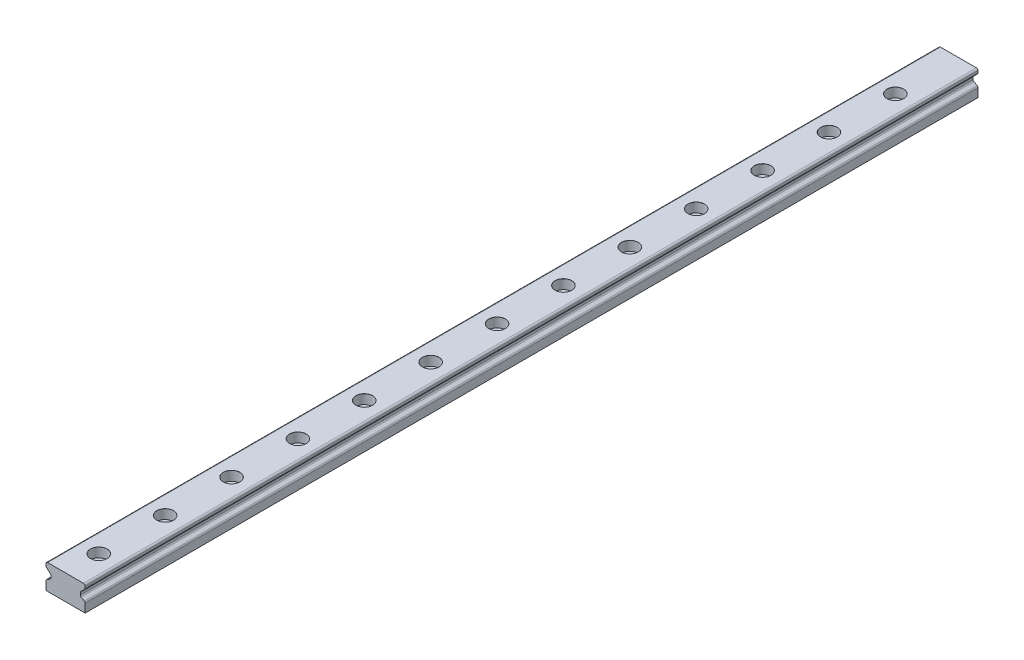
from build123d import *

# Parameters (mm, degrees)
BOSS_EXTRUDE1_DEPTH                           = 538
CBORE_FOR_M5_HEXAGON_SOCKET_HEAD_CAP_2_COUNT  = 2
CBORE_FOR_M5_HEXAGON_SOCKET_HEAD_CAP_2_PITCH  = 40
CBORE_FOR_M5_HEXAGON_SOCKET_HEAD_CAP_3_COUNT  = 2
CBORE_FOR_M5_HEXAGON_SOCKET_HEAD_CAP_3_PITCH  = 80
CBORE_FOR_M5_HEXAGON_SOCKET_HEAD_CAP_4_COUNT  = 2
CBORE_FOR_M5_HEXAGON_SOCKET_HEAD_CAP_4_PITCH  = 120
CBORE_FOR_M5_HEXAGON_SOCKET_HEAD_CAP_5_COUNT  = 2
CBORE_FOR_M5_HEXAGON_SOCKET_HEAD_CAP_5_PITCH  = 160
CBORE_FOR_M5_HEXAGON_SOCKET_HEAD_CAP_6_COUNT  = 2
CBORE_FOR_M5_HEXAGON_SOCKET_HEAD_CAP_6_PITCH  = 200
CBORE_FOR_M5_HEXAGON_SOCKET_HEAD_CAP_7_COUNT  = 2
CBORE_FOR_M5_HEXAGON_SOCKET_HEAD_CAP_7_PITCH  = 240
CBORE_FOR_M5_HEXAGON_SOCKET_HEAD_CAP_8_COUNT  = 2
CBORE_FOR_M5_HEXAGON_SOCKET_HEAD_CAP_8_PITCH  = 280
CBORE_FOR_M5_HEXAGON_SOCKET_HEAD_CAP_9_COUNT  = 2
CBORE_FOR_M5_HEXAGON_SOCKET_HEAD_CAP_9_PITCH  = 320
CBORE_FOR_M5_HEXAGON_SOCKET_HEAD_CAP_10_COUNT = 2
CBORE_FOR_M5_HEXAGON_SOCKET_HEAD_CAP_10_PITCH = 360
CBORE_FOR_M5_HEXAGON_SOCKET_HEAD_CAP_11_COUNT = 2
CBORE_FOR_M5_HEXAGON_SOCKET_HEAD_CAP_11_PITCH = 400
CBORE_FOR_M5_HEXAGON_SOCKET_HEAD_CAP_12_COUNT = 2
CBORE_FOR_M5_HEXAGON_SOCKET_HEAD_CAP_12_PITCH = 440
CBORE_FOR_M5_HEXAGON_SOCKET_HEAD_CAP_13_COUNT = 2
CBORE_FOR_M5_HEXAGON_SOCKET_HEAD_CAP_13_PITCH = 480


with BuildPart() as part:
    # Sketch1 → Boss-Extrude1 (new body)
    with BuildSketch(Plane.XY):
        with BuildLine():
            Line((-49.04910749, -219.573051322), (-49.04910749, -215.151654368))
            Line((-49.04910749, -215.151654368), (-49.04910749, -204.495232783))
            Line((-49.04910749, -204.495232783), (-59.847547756, -204.495232783))
            ThreePointArc((-59.847547756, -204.495232783), (-60.554654537, -204.788126002), (-60.847547756, -205.495232783))
            Line((-60.847547756, -205.495232783), (-60.847547756, -206.646526247))
            ThreePointArc((-60.847547756, -206.646526247), (-60.764684782, -207.045098292), (-60.529828406, -207.377616608))
            Line((-60.529828406, -207.377616608), (-58.226748647, -209.52693609))
            ThreePointArc((-58.226748647, -209.52693609), (-57.991892271, -209.859454405), (-57.909029297, -210.25802645))
            Line((-57.909029297, -210.25802645), (-57.909029297, -211.560962818))
            ThreePointArc((-57.909029297, -211.560962818), (-58.043527512, -212.061868659), (-58.410842619, -212.428032616))
            Line((-58.410842619, -212.428032616), (-60.345734434, -213.539750876))
            ThreePointArc((-60.345734434, -213.539750876), (-60.713049541, -213.905914833), (-60.847547756, -214.406820673))
            Line((-60.847547756, -214.406820673), (-60.847547756, -219.573051322))
            Line((-60.847547756, -219.573051322), (-49.04910749, -219.573051322))
        make_face()
        with BuildLine():
            Line((-49.04910749, -204.495232783), (-49.04910749, -215.151654368))
            Line((-49.04910749, -215.151654368), (-49.04910749, -219.573051322))
            Line((-49.04910749, -219.573051322), (-37.250667225, -219.573051322))
            Line((-37.250667225, -219.573051322), (-37.250667225, -214.406820673))
            ThreePointArc((-37.250667225, -214.406820673), (-37.38516544, -213.905914833), (-37.752480546, -213.539750876))
            Line((-37.752480546, -213.539750876), (-39.687372362, -212.428032616))
            ThreePointArc((-39.687372362, -212.428032616), (-40.054687468, -212.061868659), (-40.189185684, -211.560962818))
            Line((-40.189185684, -211.560962818), (-40.189185684, -210.25802645))
            ThreePointArc((-40.189185684, -210.25802645), (-40.10632271, -209.859454405), (-39.871466333, -209.52693609))
            Line((-39.871466333, -209.52693609), (-37.568386575, -207.377616608))
            ThreePointArc((-37.568386575, -207.377616608), (-37.333530198, -207.045098292), (-37.250667225, -206.646526247))
            Line((-37.250667225, -206.646526247), (-37.250667225, -205.495232783))
            ThreePointArc((-37.250667225, -205.495232783), (-37.543560443, -204.788126002), (-38.250667225, -204.495232783))
            Line((-38.250667225, -204.495232783), (-49.04910749, -204.495232783))
        make_face()
    extrude(amount=BOSS_EXTRUDE1_DEPTH)

    # Sketch3 → CBORE for M5 Hexagon socket head cap screws1 (revolve, cut)
    with BuildSketch(Plane(origin=(-49.04910749, -204.495232783, 518), x_dir=(0, 0, 1), z_dir=(1, 0, 0))):
        Polygon((0, 0), (0, 15.077818539), (2.75, 15.077818539), (2.75, 5.7), (5, 5.7), (5, 0.025), (5.025, 0), align=None)
    cbore_for_m5_hexagon_socket_head_cap_scr = revolve(axis=Axis((-49.04910749, -198.145232783, 518), (0, -1, 0)), mode=Mode.SUBTRACT)

    # CBORE for M5 Hexagon socket head cap 2: CBORE for M5 Hexagon socket head cap screws1 ×2
    with Locations(*[(0, 0, -i * CBORE_FOR_M5_HEXAGON_SOCKET_HEAD_CAP_2_PITCH) for i in range(1, CBORE_FOR_M5_HEXAGON_SOCKET_HEAD_CAP_2_COUNT)]):
        add(cbore_for_m5_hexagon_socket_head_cap_scr, mode=Mode.SUBTRACT)

    # CBORE for M5 Hexagon socket head cap 3: CBORE for M5 Hexagon socket head cap screws1 ×2
    with Locations(*[(0, 0, -i * CBORE_FOR_M5_HEXAGON_SOCKET_HEAD_CAP_3_PITCH) for i in range(1, CBORE_FOR_M5_HEXAGON_SOCKET_HEAD_CAP_3_COUNT)]):
        add(cbore_for_m5_hexagon_socket_head_cap_scr, mode=Mode.SUBTRACT)

    # CBORE for M5 Hexagon socket head cap 4: CBORE for M5 Hexagon socket head cap screws1 ×2
    with Locations(*[(0, 0, -i * CBORE_FOR_M5_HEXAGON_SOCKET_HEAD_CAP_4_PITCH) for i in range(1, CBORE_FOR_M5_HEXAGON_SOCKET_HEAD_CAP_4_COUNT)]):
        add(cbore_for_m5_hexagon_socket_head_cap_scr, mode=Mode.SUBTRACT)

    # CBORE for M5 Hexagon socket head cap 5: CBORE for M5 Hexagon socket head cap screws1 ×2
    with Locations(*[(0, 0, -i * CBORE_FOR_M5_HEXAGON_SOCKET_HEAD_CAP_5_PITCH) for i in range(1, CBORE_FOR_M5_HEXAGON_SOCKET_HEAD_CAP_5_COUNT)]):
        add(cbore_for_m5_hexagon_socket_head_cap_scr, mode=Mode.SUBTRACT)

    # CBORE for M5 Hexagon socket head cap 6: CBORE for M5 Hexagon socket head cap screws1 ×2
    with Locations(*[(0, 0, -i * CBORE_FOR_M5_HEXAGON_SOCKET_HEAD_CAP_6_PITCH) for i in range(1, CBORE_FOR_M5_HEXAGON_SOCKET_HEAD_CAP_6_COUNT)]):
        add(cbore_for_m5_hexagon_socket_head_cap_scr, mode=Mode.SUBTRACT)

    # CBORE for M5 Hexagon socket head cap 7: CBORE for M5 Hexagon socket head cap screws1 ×2
    with Locations(*[(0, 0, -i * CBORE_FOR_M5_HEXAGON_SOCKET_HEAD_CAP_7_PITCH) for i in range(1, CBORE_FOR_M5_HEXAGON_SOCKET_HEAD_CAP_7_COUNT)]):
        add(cbore_for_m5_hexagon_socket_head_cap_scr, mode=Mode.SUBTRACT)

    # CBORE for M5 Hexagon socket head cap 8: CBORE for M5 Hexagon socket head cap screws1 ×2
    with Locations(*[(0, 0, -i * CBORE_FOR_M5_HEXAGON_SOCKET_HEAD_CAP_8_PITCH) for i in range(1, CBORE_FOR_M5_HEXAGON_SOCKET_HEAD_CAP_8_COUNT)]):
        add(cbore_for_m5_hexagon_socket_head_cap_scr, mode=Mode.SUBTRACT)

    # CBORE for M5 Hexagon socket head cap 9: CBORE for M5 Hexagon socket head cap screws1 ×2
    with Locations(*[(0, 0, -i * CBORE_FOR_M5_HEXAGON_SOCKET_HEAD_CAP_9_PITCH) for i in range(1, CBORE_FOR_M5_HEXAGON_SOCKET_HEAD_CAP_9_COUNT)]):
        add(cbore_for_m5_hexagon_socket_head_cap_scr, mode=Mode.SUBTRACT)

    # CBORE for M5 Hexagon socket head cap 10: CBORE for M5 Hexagon socket head cap screws1 ×2
    with Locations(*[(0, 0, -i * CBORE_FOR_M5_HEXAGON_SOCKET_HEAD_CAP_10_PITCH) for i in range(1, CBORE_FOR_M5_HEXAGON_SOCKET_HEAD_CAP_10_COUNT)]):
        add(cbore_for_m5_hexagon_socket_head_cap_scr, mode=Mode.SUBTRACT)

    # CBORE for M5 Hexagon socket head cap 11: CBORE for M5 Hexagon socket head cap screws1 ×2
    with Locations(*[(0, 0, -i * CBORE_FOR_M5_HEXAGON_SOCKET_HEAD_CAP_11_PITCH) for i in range(1, CBORE_FOR_M5_HEXAGON_SOCKET_HEAD_CAP_11_COUNT)]):
        add(cbore_for_m5_hexagon_socket_head_cap_scr, mode=Mode.SUBTRACT)

    # CBORE for M5 Hexagon socket head cap 12: CBORE for M5 Hexagon socket head cap screws1 ×2
    with Locations(*[(0, 0, -i * CBORE_FOR_M5_HEXAGON_SOCKET_HEAD_CAP_12_PITCH) for i in range(1, CBORE_FOR_M5_HEXAGON_SOCKET_HEAD_CAP_12_COUNT)]):
        add(cbore_for_m5_hexagon_socket_head_cap_scr, mode=Mode.SUBTRACT)

    # CBORE for M5 Hexagon socket head cap 13: CBORE for M5 Hexagon socket head cap screws1 ×2
    with Locations(*[(0, 0, -i * CBORE_FOR_M5_HEXAGON_SOCKET_HEAD_CAP_13_PITCH) for i in range(1, CBORE_FOR_M5_HEXAGON_SOCKET_HEAD_CAP_13_COUNT)]):
        add(cbore_for_m5_hexagon_socket_head_cap_scr, mode=Mode.SUBTRACT)


solid = part.part
